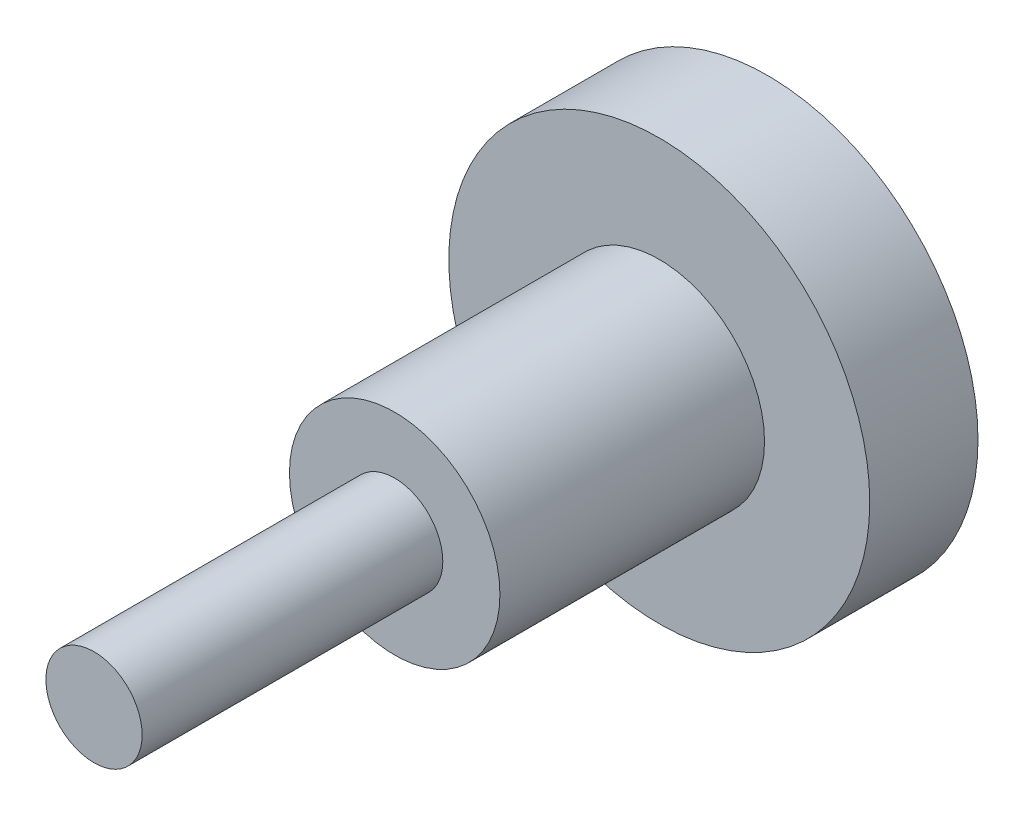
from build123d import *

# Parameters (mm, degrees)
SKETCH1_W = 8
SKETCH1_H = 50


with BuildPart() as part:
    # Sketch1 → Revolve1 (revolve)
    with BuildSketch(Plane(origin=(0, 0, 0), x_dir=(1, 0, 0), z_dir=(0, 1, 0)), mode=Mode.PRIVATE) as revolve1_sk:
        Polygon((-17.5, 94), (0, 94), (0, 112), (-35, 112), (-35, 94), align=None)
        Polygon((-8, 50), (0, 50), (0, 94), (-17.5, 94), (-17.5, 50), align=None)
        with Locations((-4, 25)):
            Rectangle(SKETCH1_W, SKETCH1_H)
    revolve(revolve1_sk.sketch.rotate(Axis((0, 0, 0), (0, 0, -1)), 180), axis=Axis((0, 0, 0), (0, 0, -1)))


solid = part.part
